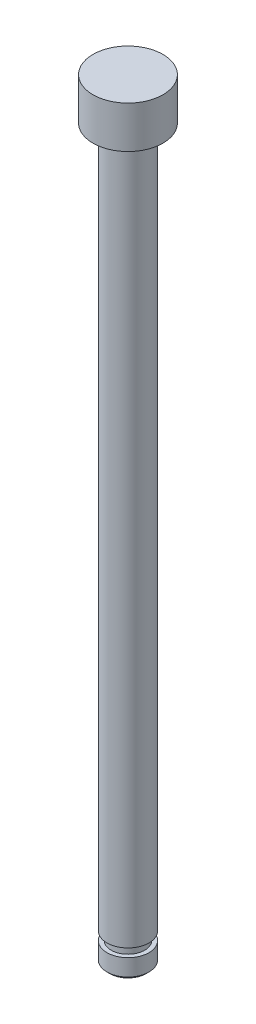
SolidWorks part; units mm, degrees
ref_plane "Front Plane" through (0, 0, 0) normal (0, 0, 1) x (1, 0, 0)
ref_plane "Top Plane" through (0, 0, 0) normal (0, 1, 0) x (1, 0, 0)
ref_plane "Right Plane" through (0, 0, 0) normal (1, 0, 0) x (0, 0, -1)
sketch "Sketch1" plane through (0, 0, 0) normal (0, 1, 0) x (1, 0, 0)
  circle A0 centre (0, 0) radius 0.75
  dimension "D1" = 1.5
extrude "Boss-Extrude1" add sketch "Sketch1" along normal blind 26
sketch "Sketch2" plane through (0, 26, 0) normal (0, 1, 0) x (1, 0, 0)
  circle A0 centre (0, 0) radius 1.25
  circle A1 centre (0, 0) radius 0.75 construction
  dimension "D1" = 0.5
extrude "Boss-Extrude2" add sketch "Sketch2" along normal blind 1.5
ref_plane "Plane1" through (0, 1, 0) normal (0, -1, 0) x (-1, 0, 0)
sketch "Sketch3" plane through (0, 1, 0) normal (0, -1, 0) x (-1, 0, 0)
  circle A0 centre (0, 0) radius 0.6
  dimension "D1" = 1.2
extrude "Cut-Extrude1" cut sketch "Sketch3" along normal blind 0.3 flip side to cut
chamfer "Chamfer1" distance 0.1 angle 45 1 edges at (0, 0, 0.75)
